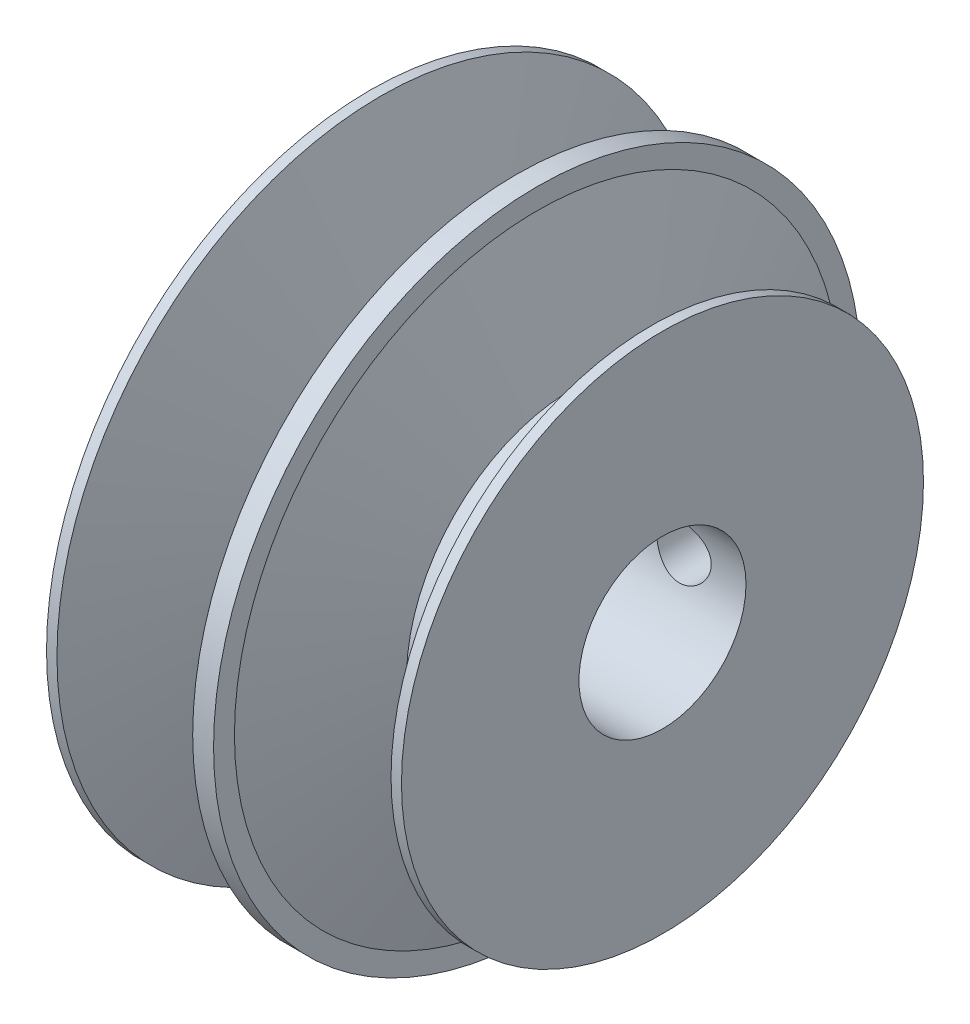
SolidWorks part; units mm, degrees
ref_plane "Front Plane" through (0, 0, 0) normal (0, 0, 1) x (1, 0, 0)
ref_plane "Top Plane" through (0, 0, 0) normal (0, 1, 0) x (1, 0, 0)
ref_plane "Right Plane" through (0, 0, 0) normal (1, 0, 0) x (0, 0, -1)
sketch "Sketch1" plane through (0, 0, 0) normal (0, 0, 1) x (1, 0, 0)
  line L0 (-65.1472, 0) -> (92.2676, 0) construction
  line L1 (-43.6103, 31) -> (-42.6103, 31)
  line L5 (-43.6103, 14) -> (-43.6103, 31)
  line L6 (-43.6103, 14) -> (-15.6103, 14)
  line L7 (-38.5911, 30.6436) -> (-38.5911, 16) construction
  line L8 (-42.6103, 31) -> (-38.5911, 16)
  line L9 (-38.5911, 16) -> (-33.6296, 16)
  line L10 (-33.6296, 16) -> (-29.6103, 31)
  line L11 (-29.6103, 31) -> (-27.6103, 31)
  line L12 (-33.6296, 16) -> (-33.6296, 40.7895) construction
  line L13 (-27.6103, 31) -> (-27.6103, 29)
  line L14 (-27.6103, 29) -> (-24.127, 16)
  line L15 (-27.6103, 29) -> (-27.6103, 18.3389) construction
  line L16 (-42.6103, 31) -> (-42.6103, 17.1275) construction
  line L17 (-24.127, 16) -> (-19.0219, 16)
  line L18 (-19.0219, 16) -> (-16.6103, 25)
  line L19 (-16.6103, 25) -> (-15.6103, 25)
  line L20 (-15.6103, 25) -> (-15.6103, 14)
  point P3 (0, 0)
  dimension "D2" = 1
  dimension "D3" = 2
  dimension "D4" = 16
  dimension "D5" = 16
  dimension "D6" = 2
  dimension "D7" = 15
  dimension "D8" = 12
  dimension "D9" = 1
  dimension "D10" = 16
  dimension "D11" = 25
  dimension "D12" = 15
  dimension "D13" = 14
  dimension "D14" = 31
  dimension "D15" = 31
  dimension "D16" = 15
revolve "Revolve1" add sketch "Sketch1" angle 360 about L0
sketch "Sketch2" plane through (-15.6103, 0, 0) normal (1, 0, 0) x (0, 0, -1)
  circle A0 centre (0, 0) radius 14.8547
  circle A1 centre (0, 0) radius 8
  dimension "D1" = 16
extrude "Boss-Extrude1" add sketch "Sketch2" against normal through all
sketch "Sketch3" plane through (-43.6103, 0, 0) normal (-1, 0, 0) x (0, 0, 1)
  circle A0 centre (0, 0) radius 14
  dimension "D1" = 28
extrude "Cut-Extrude1" cut sketch "Sketch3" against normal up to surface (16 mm away) up to face at (-27.6103, 0, 31)
sketch "Sketch4" plane through (0, 0, 0) normal (0, 1, 0) x (1, 0, 0)
  line L0 (0, 0) -> (-21.5744, 0) construction
  line L1 (-21.5744, 16) -> (-21.5744, 0) construction
  line L2 (-19.0219, 16) -> (-24.127, 16) construction
  circle A0 centre (-21.5744, 0) radius 2.5
  dimension "D1" = 5
hole_wizard "#5 (0.2055) Diameter Hole1" positions "3DSketch1" profile "Sketch6" hole size "#5" standard "ANSI Inch"
sketch3d "3DSketch1"
  point P0 (-21.5744, 0, 0)
  point P3 (-21.5744, 0, 0)
  point P5 (-21.5744, 0, 0)
  point P7 (-21.5744, 0, 0)
  point P9 (-21.5481, 0.0429, 15.9999)
  point P12 (-21.5744, 0, 0)
sketch "Sketch6" plane through (-21.5481, 0.0429, 15.9999) normal (1, 0, 0) x (0, -1, 0.0027)
  line L0 (0, 0) -> (0, 47.0829)
  line L1 (0, 47.0829) -> (2.6098, 47.0829)
  line L2 (2.6098, 47.0829) -> (2.6098, 0)
  line L5 (2.6098, 0) -> (0, 0)
  line L11 (0, -6.35) -> (0, 107.95) construction
  dimension "Thru Hole Dia." = 5.2197
  dimension "Thru Hole Depth" = 47.0829
